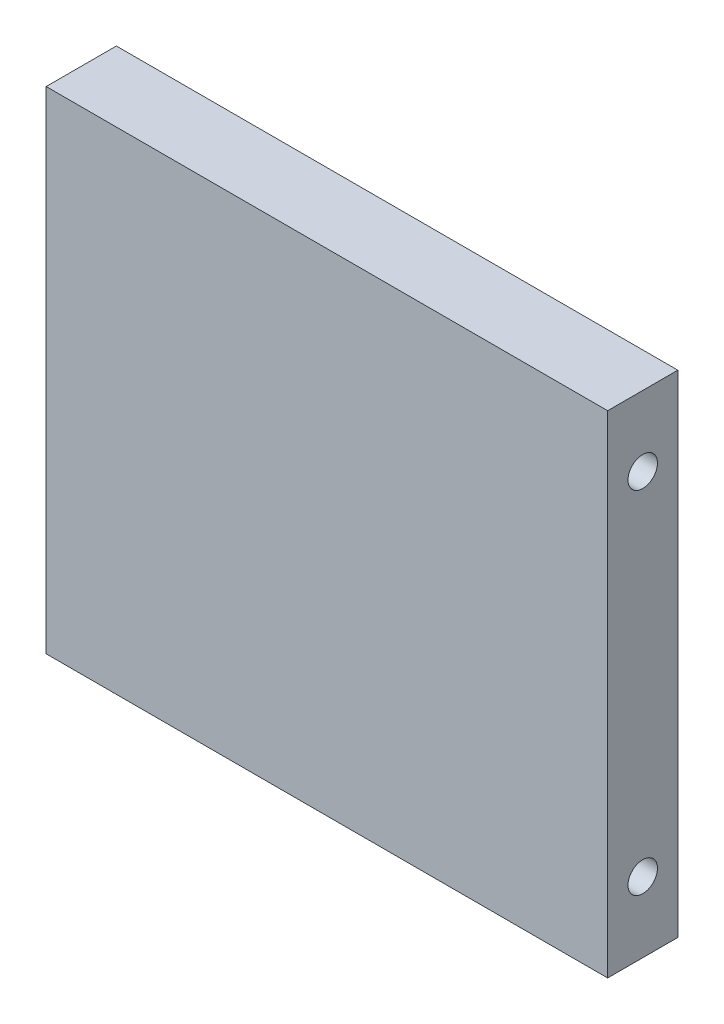
from build123d import *

# Parameters (mm, degrees)
SKETCH_1_W             = 80
SKETCH_1_H             = 70
EXTRUDE_1_DEPTH        = 10
HOLE_WIZARD_M5_1_D     = 4.2
HOLE_WIZARD_M5_1_DEPTH = 14
HOLE_WIZARD_M5_1_TIP   = 1.2618073
HOLE_WIZARD_M5_2_D     = 4.2
HOLE_WIZARD_M5_2_DEPTH = 14
HOLE_WIZARD_M5_2_TIP   = 1.2618073


with BuildPart() as part:
    # 草图1 → 凸台-拉伸1 (new body)
    with BuildSketch(Plane.XY):
        Rectangle(SKETCH_1_W, SKETCH_1_H)
    extrude(amount=EXTRUDE_1_DEPTH)

    # M5 螺纹孔1
    with Locations(Plane(origin=(40, 0, 0), x_dir=(0, 0, -1), z_dir=(1, 0, 0))):
        with Locations((-5, -25), (-5, 25)):
            Hole(HOLE_WIZARD_M5_1_D / 2, depth=HOLE_WIZARD_M5_1_DEPTH)
            with Locations((0, 0, -(HOLE_WIZARD_M5_1_DEPTH + HOLE_WIZARD_M5_1_TIP / 2))):  # 118° drill point
                Cone(0, HOLE_WIZARD_M5_1_D / 2, HOLE_WIZARD_M5_1_TIP, mode=Mode.SUBTRACT)

    # M5 螺纹孔2
    with Locations(Plane.ZY.offset(40)):
        with Locations((5, 25), (5, -25)):
            Hole(HOLE_WIZARD_M5_2_D / 2, depth=HOLE_WIZARD_M5_2_DEPTH)
            with Locations((0, 0, -(HOLE_WIZARD_M5_2_DEPTH + HOLE_WIZARD_M5_2_TIP / 2))):  # 118° drill point
                Cone(0, HOLE_WIZARD_M5_2_D / 2, HOLE_WIZARD_M5_2_TIP, mode=Mode.SUBTRACT)


solid = part.part
